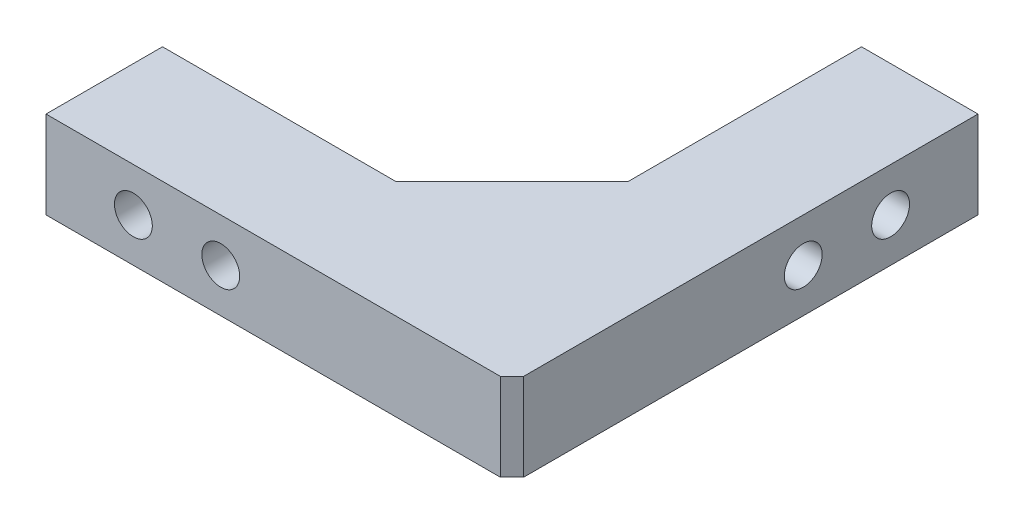
from build123d import *

# Parameters (mm, degrees)
BOSS_EXTRUDE_1_DEPTH   = 15
SKETCH_4_R             = 3.25
CUT_EXTRUDE_1_DEPTH    = 74.654599313
LINEAR_PATTERN_1_COUNT = 2
LINEAR_PATTERN_1_PITCH = 15
SKETCH_5_R             = 3.25
CUT_EXTRUDE_2_DEPTH    = 91.691785736
LINEAR_PATTERN_2_COUNT = 2
LINEAR_PATTERN_2_PITCH = 15
CHAMFER_1_SIZE         = 2


with BuildPart() as part:
    # Sketch 3 → Boss-Extrude 1 (new body)
    with BuildSketch(Plane(origin=(0, 0, 0), x_dir=(1, 0, 0), z_dir=(0, 1, 0))):
        Polygon((40, 40), (20, 40), (20, 0), (0, -20), (-40, -20), (-40, -40), (40, -40), align=None)
    extrude(amount=BOSS_EXTRUDE_1_DEPTH)

    # Sketch 4 → Cut-Extrude 1 (cut, through all)
    with BuildSketch(Plane(origin=(0, 0, 20), x_dir=(-1, 0, 0), z_dir=(0, 0, -1))):
        with Locations((10, 7.5)):
            Circle(SKETCH_4_R)
    cut_extrude_1 = extrude(amount=-CUT_EXTRUDE_1_DEPTH, mode=Mode.SUBTRACT)

    # Linear Pattern 1: Cut-Extrude 1 ×2
    with Locations(*[(-i * LINEAR_PATTERN_1_PITCH, 0, 0) for i in range(1, LINEAR_PATTERN_1_COUNT)]):
        add(cut_extrude_1, mode=Mode.SUBTRACT)

    # Sketch 5 → Cut-Extrude 2 (cut, through all)
    with BuildSketch(Plane(origin=(40, 0, 0), x_dir=(0, 0, -1), z_dir=(1, 0, 0))):
        with Locations((10, 7.5)):
            Circle(SKETCH_5_R)
    cut_extrude_2 = extrude(amount=-CUT_EXTRUDE_2_DEPTH, mode=Mode.SUBTRACT)

    # Linear Pattern 2: Cut-Extrude 2 ×2
    with Locations(*[(0, 0, -i * LINEAR_PATTERN_2_PITCH) for i in range(1, LINEAR_PATTERN_2_COUNT)]):
        add(cut_extrude_2, mode=Mode.SUBTRACT)

    # Chamfer 1
    chamfer_1_edges = [part.edges().sort_by_distance(p)[0] for p in [
        (40, 7.5, 40),
    ]]
    chamfer(chamfer_1_edges, length=CHAMFER_1_SIZE)


solid = part.part
